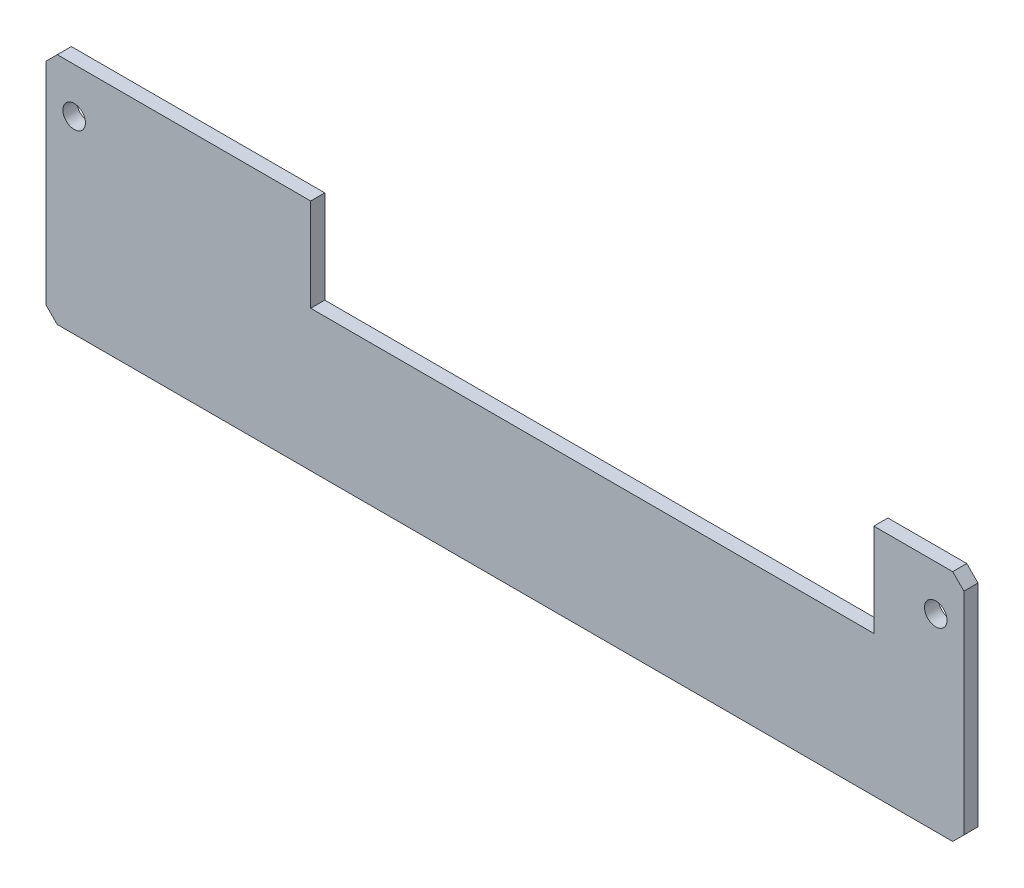
from build123d import *

# Parameters (mm, degrees)
SKETCH1_W               = 1630
SKETCH1_H               = 415
BOSS_EXTRUDE1_DEPTH     = 25
CHAMFER1_SIZE           = 20
CUT_EXTRUDE1_DEPTH      = 842.371647965
CUT_EXTRUDE1_DEPTH_BACK = 842.371647965
SKETCH2_R               = 20
SKETCH2_W               = 1000
SKETCH2_H               = 200


with BuildPart() as part:
    # Sketch1 → Boss-Extrude1 (new body)
    with BuildSketch(Plane.XY):
        Rectangle(SKETCH1_W, SKETCH1_H)
    extrude(amount=BOSS_EXTRUDE1_DEPTH)

    # Chamfer1
    chamfer1_edges = [part.edges().sort_by_distance(p)[0] for p in [
        (-815, 207.5, 12.5),
        (815, 207.5, 12.5),
        (815, -207.5, 12.5),
        (-815, -207.5, 12.5),
    ]]
    chamfer(chamfer1_edges, length=CHAMFER1_SIZE)

    # Sketch2 → Cut-Extrude1 (cut, two sides: drawn at the far end of the back side and taken through both)
    with BuildSketch(Plane.XY.offset(25).offset(-CUT_EXTRUDE1_DEPTH_BACK)):
        with Locations((-765, 127.5)):
            Circle(SKETCH2_R)
        with Locations((765, 127.5)):
            Circle(SKETCH2_R)
        with Locations((155, 142.5)):
            Rectangle(SKETCH2_W, SKETCH2_H)
    extrude(amount=CUT_EXTRUDE1_DEPTH + CUT_EXTRUDE1_DEPTH_BACK, mode=Mode.SUBTRACT)


solid = part.part
